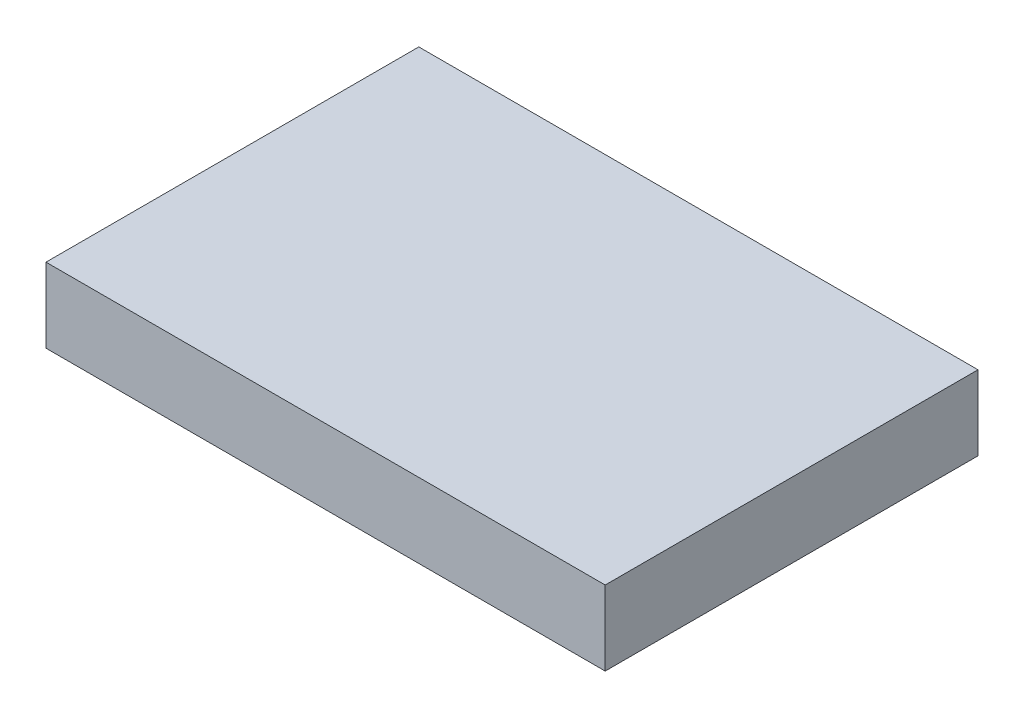
SolidWorks part; units mm, degrees
ref_plane "前视基准面" through (0, 0, 0) normal (0, 0, 1) x (1, 0, 0)
ref_plane "上视基准面" through (0, 0, 0) normal (0, 1, 0) x (1, 0, 0)
ref_plane "右视基准面" through (0, 0, 0) normal (1, 0, 0) x (0, 0, -1)
sketch "草图1" plane through (0, 0, 0) normal (0, 1, 0) x (1, 0, 0)
  line L1 (-37.5, -25) -> (37.5, -25)
  line L2 (-37.5, -25) -> (-37.5, 25)
  line L3 (-37.5, 25) -> (37.5, 25)
  line L4 (37.5, -25) -> (37.5, 25)
  line L5 (-37.5, -25) -> (37.5, 25) construction
  line L6 (-37.5, 25) -> (37.5, -25) construction
  point P0 (0, 0)
  dimension "D1" = 50
  dimension "D2" = 75
extrude "凸台-拉伸1" add sketch "草图1" along normal blind 10
